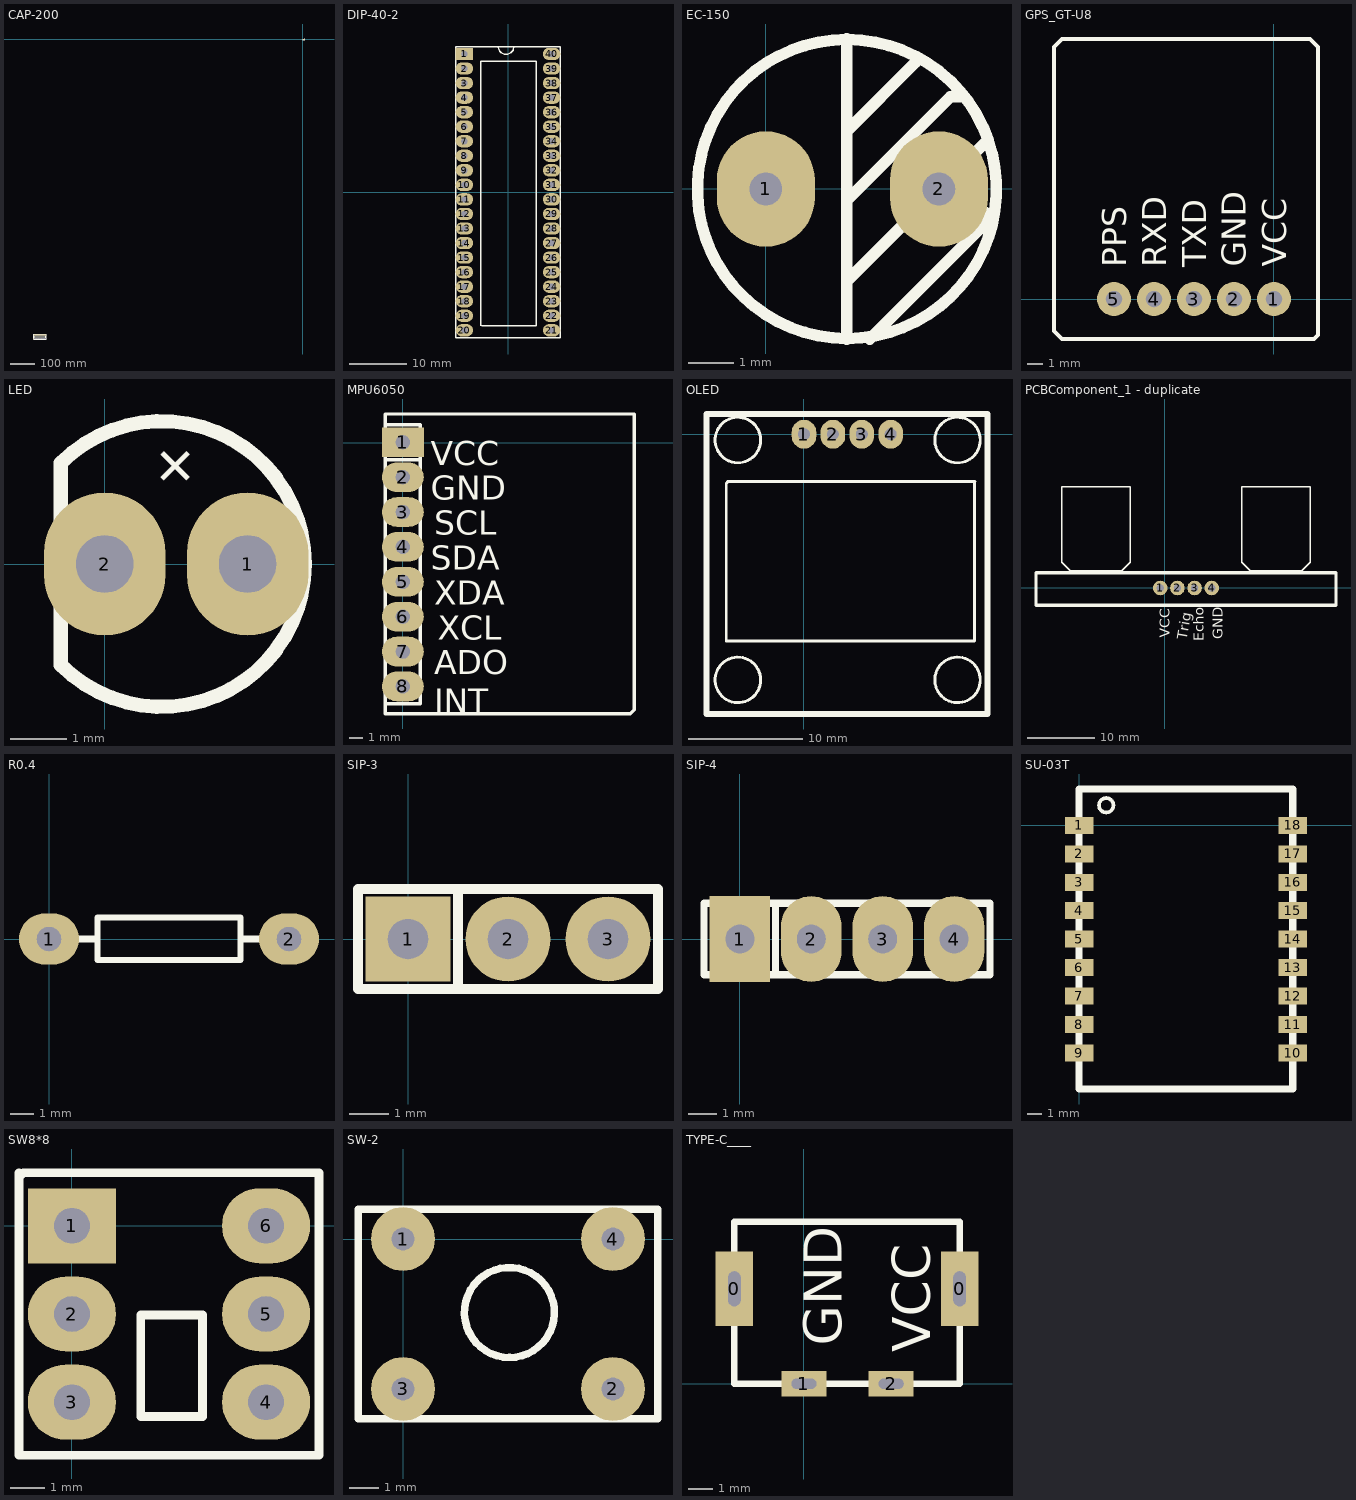
[diagram p0: the footprints below, top view; thin cyan lines are the x and y axes]
# Altium footprint library MISC80722-2.PcbLib: 15 footprints
Each footprint in its own frame and in the unit in brackets; x right, y up, seen from the top. Pads: shape width x height; smd on the part's side, far side on the other; paste and mask are expansions set on the pad; w line width, h text height; cw(c..) or ccw(c..) is an arc to the next point about the centre after c.

## CAP-200 [mil]
pads (42):
  rect 85x120 hole 40 slot 40.2 at 90 deg paste+0 mask+2: 1(-42930,-47788)
  oval 85x100 hole 30 slot 30.2 at 90 deg paste+0 mask+2: 1(0,0) 2(200,0)
  oval 85x120 hole 40 slot 40.2 at 90 deg paste+0 mask+2: 2(-42830,-47788) 3(-42730,-47788) 4(-42630,-47788) 5(-42530,-47788) 6(-42430,-47788) 7(-42330,-47788) 8(-42230,-47788) 9(-42130,-47788) 10(-42030,-47788) 11(-41930,-47788) 12(-41830,-47788) 13(-41730,-47788) 14(-41630,-47788) 15(-41530,-47788) 16(-41430,-47788) 17(-41330,-47788) 18(-41230,-47788) 19(-41130,-47788) 20(-41030,-47788) 21(-41030,-47188) 22(-41130,-47188) 23(-41230,-47188) 24(-41330,-47188) 25(-41430,-47188) 26(-41530,-47188) 27(-41630,-47188) 28(-41730,-47188) 29(-41830,-47188) 30(-41930,-47188) 31(-42030,-47188) 32(-42130,-47188) 33(-42230,-47188) 34(-42330,-47188) 35(-42430,-47188) 36(-42530,-47188) 37(-42630,-47188) 38(-42730,-47188) 39(-42830,-47188) 40(-42930,-47188)
Top Overlay:
  lines w10: -42980,-47554 ccw(c-42980,-47501) -42980,-47448 ; -41060,-47673.98 -42880,-47673.98 -42880,-47293.98 -41060,-47293.98 -41060,-47668 ; -42980,-47848 -40980,-47848 -40980,-47128 -42980,-47128 -42980,-47848 ; 0,-60 cw(c0,0) 0,60 200,60 cw(c200,0) 200,-60 0,-60

## DIP-40-2 [mil]
pads (40):
  rect 120x85 hole 40 slot 40.2 at 0 deg paste+0 mask+2: 1(-300,950)
  oval 120x85 hole 40 slot 40.2 at 0 deg paste+0 mask+2: 2(-300,850) 3(-300,750) 4(-300,650) 5(-300,550) 6(-300,450) 7(-300,350) 8(-300,250) 9(-300,150) 10(-300,50) 11(-300,-50) 12(-300,-150) 13(-300,-250) 14(-300,-350) 15(-300,-450) 16(-300,-550) 17(-300,-650) 18(-300,-750) 19(-300,-850) 20(-300,-950) 21(300,-950) 22(300,-850) 23(300,-750) 24(300,-650) 25(300,-550) 26(300,-450) 27(300,-350) 28(300,-250) 29(300,-150) 30(300,-50) 31(300,50) 32(300,150) 33(300,250) 34(300,350) 35(300,450) 36(300,550) 37(300,650) 38(300,750) 39(300,850) 40(300,950)
Top Overlay:
  lines w10: -185.98,-920 -185.98,900 194.02,900 194.02,-920 -180,-920 ; -66,1000 ccw(c-13,1000) 40,1000 ; -360,-1000 360,-1000 360,1000 -360,1000 -360,-1000

## EC-150 [mil]
pads (2):
  oval 85x100 hole 28 slot 28.2 at 90 deg paste+0 mask+2: 1(0,0) 2(150,0)
Top Overlay:
  lines w10: 70,-130 70,130 ; 70,-80 80,-70 190,40 ; 70,-10 160,80 170,80 ; 70,50 130,110 ; 70.1,-129.58 cw(c70.26,0) 70.42,-129.58 ; 90,-130 190,-30 190,-20

## GPS_GT-U8 [mil]
pads (5):
  round 85 hole 40 slot 40.2 at 0 deg paste+0 mask+2: 1(0,0) 2(-100,0) 3(-200,0) 4(-300,0) 5(-400,0)
Top Overlay:
  lines w10: -550,280 -550,-80 ; -550,-80 -530,-100 -520,-100 -500,-100 100,-100 110,-90 110,630 90,650 -530,650 -550,630 -550,628.66 -550,-80
  text "PPS" at -370,80 h60
  text "RXD" at -270,80 h60
  text "TXD" at -170,80 h60
  text "GND" at -70,80 h60
  text "VCC" at 30,80 h60

## LED [mil]
pads (2):
  oval 85x100 hole 40 slot 40.2 at 90 deg paste+0 mask+2: 1(100,0) 2(0,0)
Top Overlay:
  lines w10: -30.71,-70.71 ccw(c40,0) -30.71,70.71 -30.71,-70.71
  text "+" at 70.61,65.61 h30

## MPU6050 [mil]
pads (8):
  rect 120x85 hole 40 slot 40.2 at 0 deg paste+0 mask+2: 1(0,1)
  oval 120x85 hole 40 slot 40.2 at 0 deg paste+0 mask+2: 2(0,-99) 3(0,-199) 4(0,-299) 5(0,-399) 6(0,-499) 7(0,-599) 8(0,-699)
Top Overlay:
  lines w10: -50,-49 50,-49 ; -49,81 -50,82 ; -50,-749 -50,-778 -49,-777 560,-777 652,-777 663,-766 663,82 -50,82 ; -50,-749 50,-749 50,51 -50,51 ; -50,-749 -50,51 ; -50,51 -50,82
  text "INT" at 90,-774.48 h68.97
  text "ADO" at 90,-664.48 h68.97
  text "XCL" at 100,-564.48 h68.97
  text "XDA" at 90,-464.48 h68.97
  text "SDA" at 80,-364.48 h68.97
  text "SCL" at 90,-264.48 h68.97
  text "GND" at 80,-164.48 h68.97
  text "VCC" at 80,-64.48 h68.97

## OLED [mil]
pads (4):
  oval 85x100 hole 40 slot 40.2 at 90 deg paste+0 mask+2: 1(0,0) 2(100,0) 3(200,0) 4(300,0)
Top Overlay:
  lines w10: -150,-850.19 cw(c-228.74,-850.1) -150,-850 ; -150,-20.19 cw(c-228.74,-20.1) -150,-20 ; 610,-850.19 cw(c531.26,-850.1) 610,-850 ; 610,-20.19 cw(c531.26,-20.1) 610,-20 ; -269,-715 -269,-170 -262,-163 591,-163 590,-164 590,-715 -269,-715
  lines w20: -337.44,-967.99 635,-967.99 635,70 -337.44,70 -337.44,-967.99

## PCBComponent_1 - duplicate [mil]
pads (4):
  round 85 hole 40 slot 40.2 at 0 deg paste+0 mask+2: 1(-25,0) 2(75,0) 3(175,0) 4(275,0)
Top Overlay:
  lines w10: -600,588.98 -600,150 -550,100 -250,100 -200,150 -200,588.98 ; -600,590 -200,590 ; 450,588.98 450,150 500,100 800,100 850,150 850,588.98 ; 450,590 850,590
  lines w20: -750,-100 -750,90 1000,90 1000,-100 -750,-100
  text "VCC" at 30,-290 h60
  text "Trig" at 129.54,-305.21 h60
  text "Echo" at 230,-310 h60
  text "GND" at 340,-300 h60

## R0.4 [mil]
pads (2):
  oval 100x85 hole 40 slot 40.2 at 0 deg paste+0 mask+2: 1(0,0) 2(400,0)
Top Overlay:
  lines w10: 81,-35 319,-35 319,36 81,36 81,-35
  lines w12: 40,0 80,0 ; 320,0 360,0

## SIP-3 [mil]
pads (3):
  rect 85x85 hole 40 slot 40.2 at 0 deg paste+0 mask+2: 1(0,0)
  round 85 hole 40 slot 40.2 at 0 deg paste+0 mask+2: 2(100,0) 3(200,0)
Top Overlay:
  lines w10: 50,-50 50,50 ; -50,-50 -50,50 250,50 250,-50 -50,-50

## SIP-4 [mil]
pads (4):
  rect 85x120 hole 40 slot 40.2 at 90 deg paste+0 mask+2: 1(0,0)
  oval 85x120 hole 40 slot 40.2 at 90 deg paste+0 mask+2: 2(100,0) 3(200,0) 4(300,0)
Top Overlay:
  lines w10: 50,-50 50,50 ; -50,-50 -50,50 350,50 350,-50 -50,-50

## SU-03T [mm]
pads (18):
  rect 2x1.2 smd paste+0 mask+0.051: 1(0,-0.016) 2(0,-2.016) 3(0,-4.016) 4(0,-5.986) 5(0,-7.986) 6(0,-9.986) 7(0,-11.986) 8(0,-13.986) 9(0,-15.986) 10(15,-15.986) 11(15,-13.986) 12(15,-11.986) 13(15,-9.986) 14(15,-7.986) 15(15,-5.986) 16(15,-4.016) 17(15,-2.016) 18(15,-0.016)
Top Overlay:
  lines w0.254: 1.9,0.889 cw(c1.905,1.397) 1.905,0.889
  lines w0.508: 0,-18.5 0,2.5 ; 0.002,-18.5 14.986,-18.5 14.986,2.5 ; 0.002,2.54 14.986,2.54

## SW8*8 [mil]
pads (6):
  rect 100x85 hole 40 slot 40.2 at 0 deg paste+0 mask+2: 1(0,0)
  oval 100x85 hole 40 slot 40.2 at 0 deg paste+0 mask+2: 2(0,-100) 3(0,-200) 4(220,-200) 5(220,-100) 6(220,0)
Top Overlay:
  lines w10: -60,55 -55,60 280,60 280,-260 -60,-260 -60,60 ; 78,-216 78,-101 148,-101 148,-216 78,-216

## SW-2 [mil]
pads (4):
  round 85 hole 30 slot 30.2 at 0 deg paste+0 mask+2: 1(0,0) 2(280,-200) 3(0,-200) 4(280,0)
Top Overlay:
  lines w10: 141.85,-158 cw(c141.93,-98) 142,-158 ; -60,-240 -60,40 340,40 340,-240 -60,-240

## TYPE-C____ [mm]
pads (4):
  rect 1.5x3 hole 0.5 slot 1.4 at 90 deg paste+0 mask+0.051: 0(-2.794,3.81) 0(6.25,3.81)
  rect 1.8x1.016 hole 0.4 slot 1 at 0 deg paste+0 mask+0.051: 1(0,0) 2(3.5,0)
Top Overlay:
  lines w0.254: -2.794,0 -2.794,6.5 6.25,6.5 6.25,0 -2.794,0
  text "VCC" at 5.08,1.27 h1.52
  text "GND" at 1.524,1.524 h1.52
Bottom Overlay:
  text "GND" at -1.524,1.524 h1.52
  text "VCC" at 2.032,1.27 h1.52